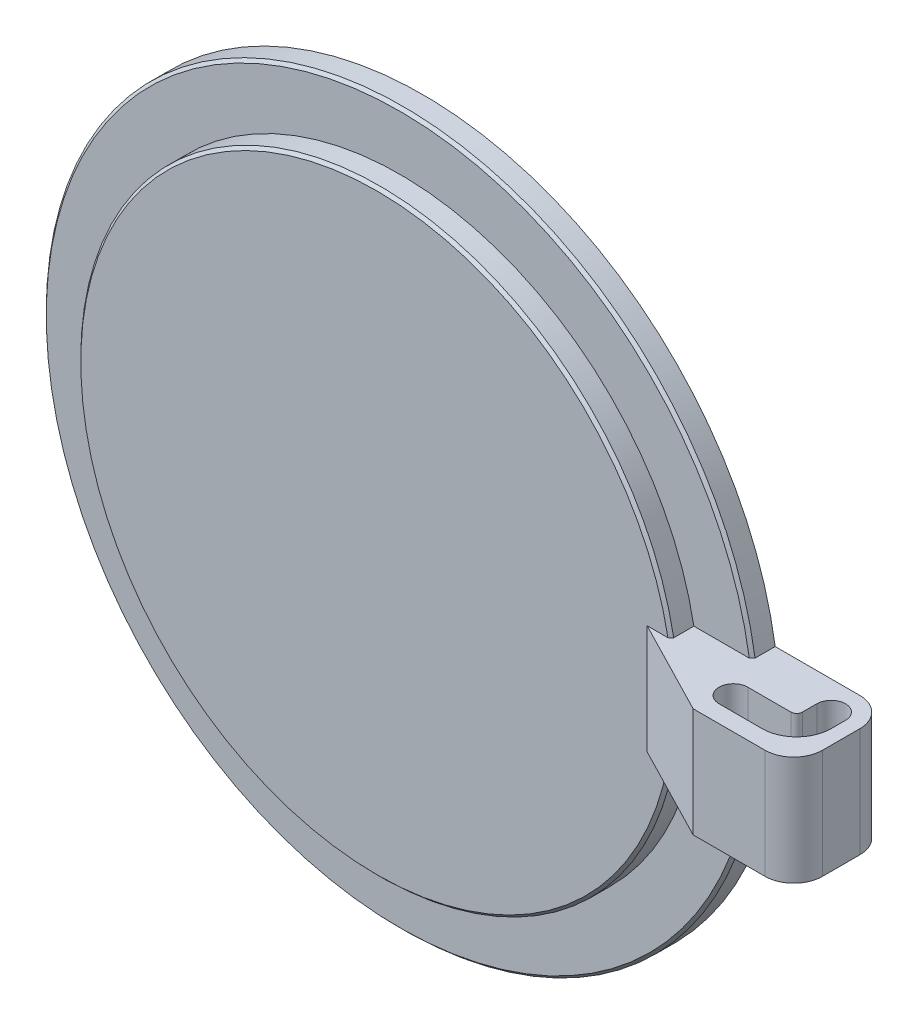
SolidWorks part; units mm, degrees
ref_plane "前视基准面" through (0, 0, 0) normal (0, 0, 1) x (1, 0, 0)
ref_plane "上视基准面" through (0, 0, 0) normal (0, 1, 0) x (1, 0, 0)
ref_plane "右视基准面" through (0, 0, 0) normal (1, 0, 0) x (0, 0, -1)
sketch "草图1" plane through (0, 0, 0) normal (0, 0, 1) x (1, 0, 0)
  circle A0 centre (0, 0) radius 62
  dimension "D1" = 124
extrude "凸台-拉伸1" add sketch "草图1" along normal blind 4
sketch "草图2" plane through (0, 0, 4) normal (0, 0, 1) x (1, 0, 0)
  circle A0 centre (0, 0) radius 52
  dimension "D1" = 104
extrude "凸台-拉伸2" add sketch "草图2" along normal blind 4
sketch "草图3" plane through (0, 0, 0) normal (0, 1, 0) x (1, 0, 0)
  line L0 (81, 0) -> (81, -11.5)
  line L1 (65, -11) -> (76, -11) construction
  line L2 (76, -16.5) -> (63.5, -16.5)
  line L3 (63.5, -16.5) -> (47, -8)
  line L4 (-52, -8) -> (52, -8) construction
  line L5 (47, -8) -> (47, 0)
  line L6 (62, 0) -> (-62, 0) construction
  line L7 (47, 0) -> (81, 0)
  line L8 (73.5, -5) -> (73.5, -7.5)
  line L9 (65, -8.5) -> (72.5, -8.5)
  line L10 (65, -13.5) -> (72.5, -13.5)
  line L11 (76, -11) -> (76, -1.2737) construction
  line L14 (78.5, -5) -> (78.5, -7.5)
  arc A0 (65, -8.5) -> (65, -13.5) centre (65, -11) ccw
  arc A1 (78.5, -7.5) -> (72.5, -13.5) centre (72.5, -7.5) cw
  arc A2 (78.5, -5) -> (73.5, -5) centre (76, -5) ccw
  arc A3 (73.5, -7.5) -> (72.5, -8.5) centre (72.5, -7.5) cw
  arc A4 (81, -11.5) -> (76, -16.5) centre (76, -11.5) cw
  point P5 (70.5, -11)
  point P14 (78.0723, -13.5)
  point P17 (78.1281, -13.5)
  dimension "D3" = 5
  dimension "D4" = 3
  dimension "D5" = 65
  dimension "D6" = 5
  dimension "D7" = 5
  dimension "D8" = 5
  dimension "D9" = 2.5
  dimension "D10" = 6
  dimension "D11" = 1
  dimension "D12" = 5
  dimension "D1" = 16.5
  dimension "D2" = 81
extrude "凸台-拉伸3" add sketch "草图3" along normal mid plane 19
fillet "圆角1" radius 5 1 edges at (81, 0, 0)
chamfer "倒角1" distance 0.5 angle 45 2 edges at (-62, 0, 4) (-52, 0, 8)
